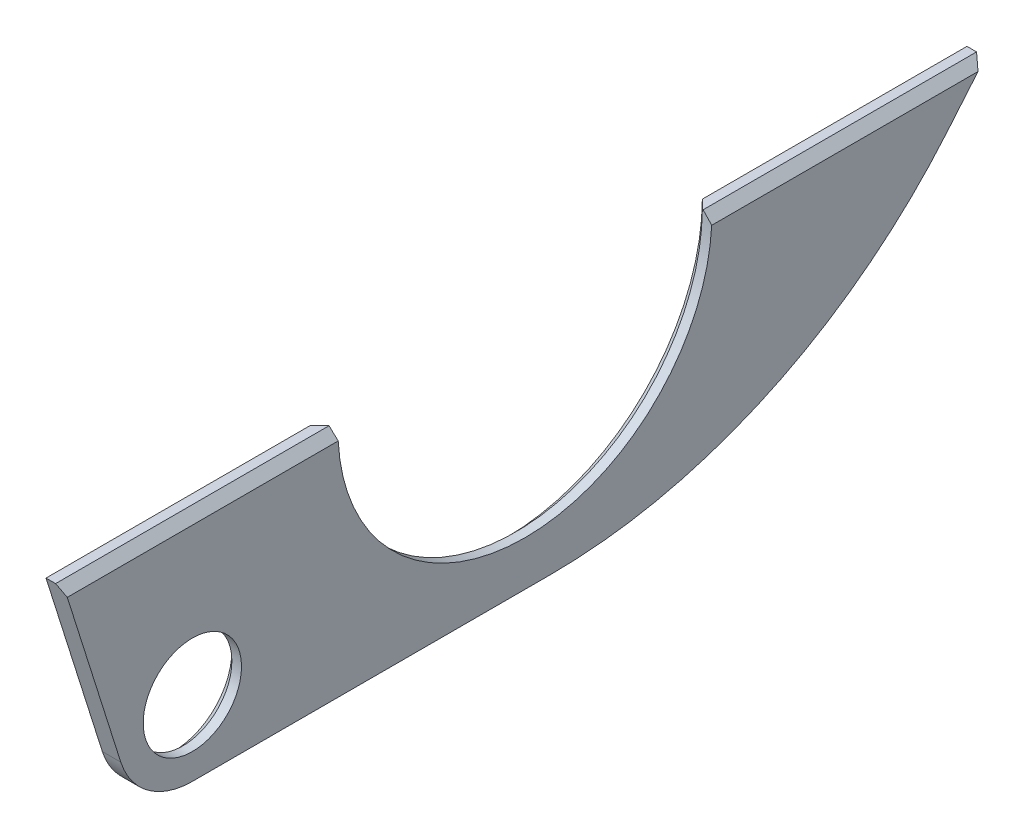
SolidWorks part; units mm, degrees
material "Q345B"
ref_plane "Front Plane" through (0, 0, 0) normal (0, 0, 1) x (1, 0, 0)
ref_plane "Top Plane" through (0, 0, 0) normal (0, 1, 0) x (1, 0, 0)
ref_plane "Right Plane" through (0, 0, 0) normal (1, 0, 0) x (0, 0, -1)
sketch "Sketch1" plane through (0, 0, 0) normal (1, 0, 0) x (0, 0, -1)
  line L0 (-55.2907, 0) -> (73.0254, 0) construction
  line L1 (0, 67.5426) -> (0, -31.3548) construction
  line L2 (623, -1.2) -> (252.9972, -1.2)
  line L3 (-623, -1.2) -> (-546.7897, -242.5615)
  line L6 (-450, -313.5) -> (360.9492, -313.5)
  line L7 (360.9492, -313.5) -> (623, -1.2)
  line L11 (-252.9972, -1.2) -> (-623, -1.2)
  arc A0 (-252.9972, -1.2) -> (252.9972, -1.2) centre (0, 0) ccw
  arc A2 (-546.7897, -242.5615) -> (-450, -313.5) centre (-450, -212) ccw
  dimension "D1" = 506
  dimension "D2" = 101.5
  dimension "D3" = 50
  dimension "D4" = 623
  dimension "D5" = 1.2
  dimension "D6" = 623
  dimension "D14" = 450
  dimension "D15" = 212
extrude "Boss-Extrude1" add sketch "Sketch1" along normal mid plane 25
sketch "Sketch2" plane through (0, 0, 0) normal (1, 0, 0) x (0, 0, -1)
  circle A1 centre (-450, -212) radius 66.5
  dimension "D1" = 133
extrude "Cut-Extrude1" cut sketch "Sketch2" against normal through all both and the other way through all
fillet "Fillet1" radius 700 1 edges at (0, -313.5, -360.9492)
chamfer "Chamfer1" distance 12 angle 45 2 edges at (-12.5, -212, 383.5) (-12.5, -253, 0)
chamfer "Chamfer2" distance 12 angle 45 2 edges at (12.5, -1.2, -437.9986) (12.5, -1.2, 437.9986)
